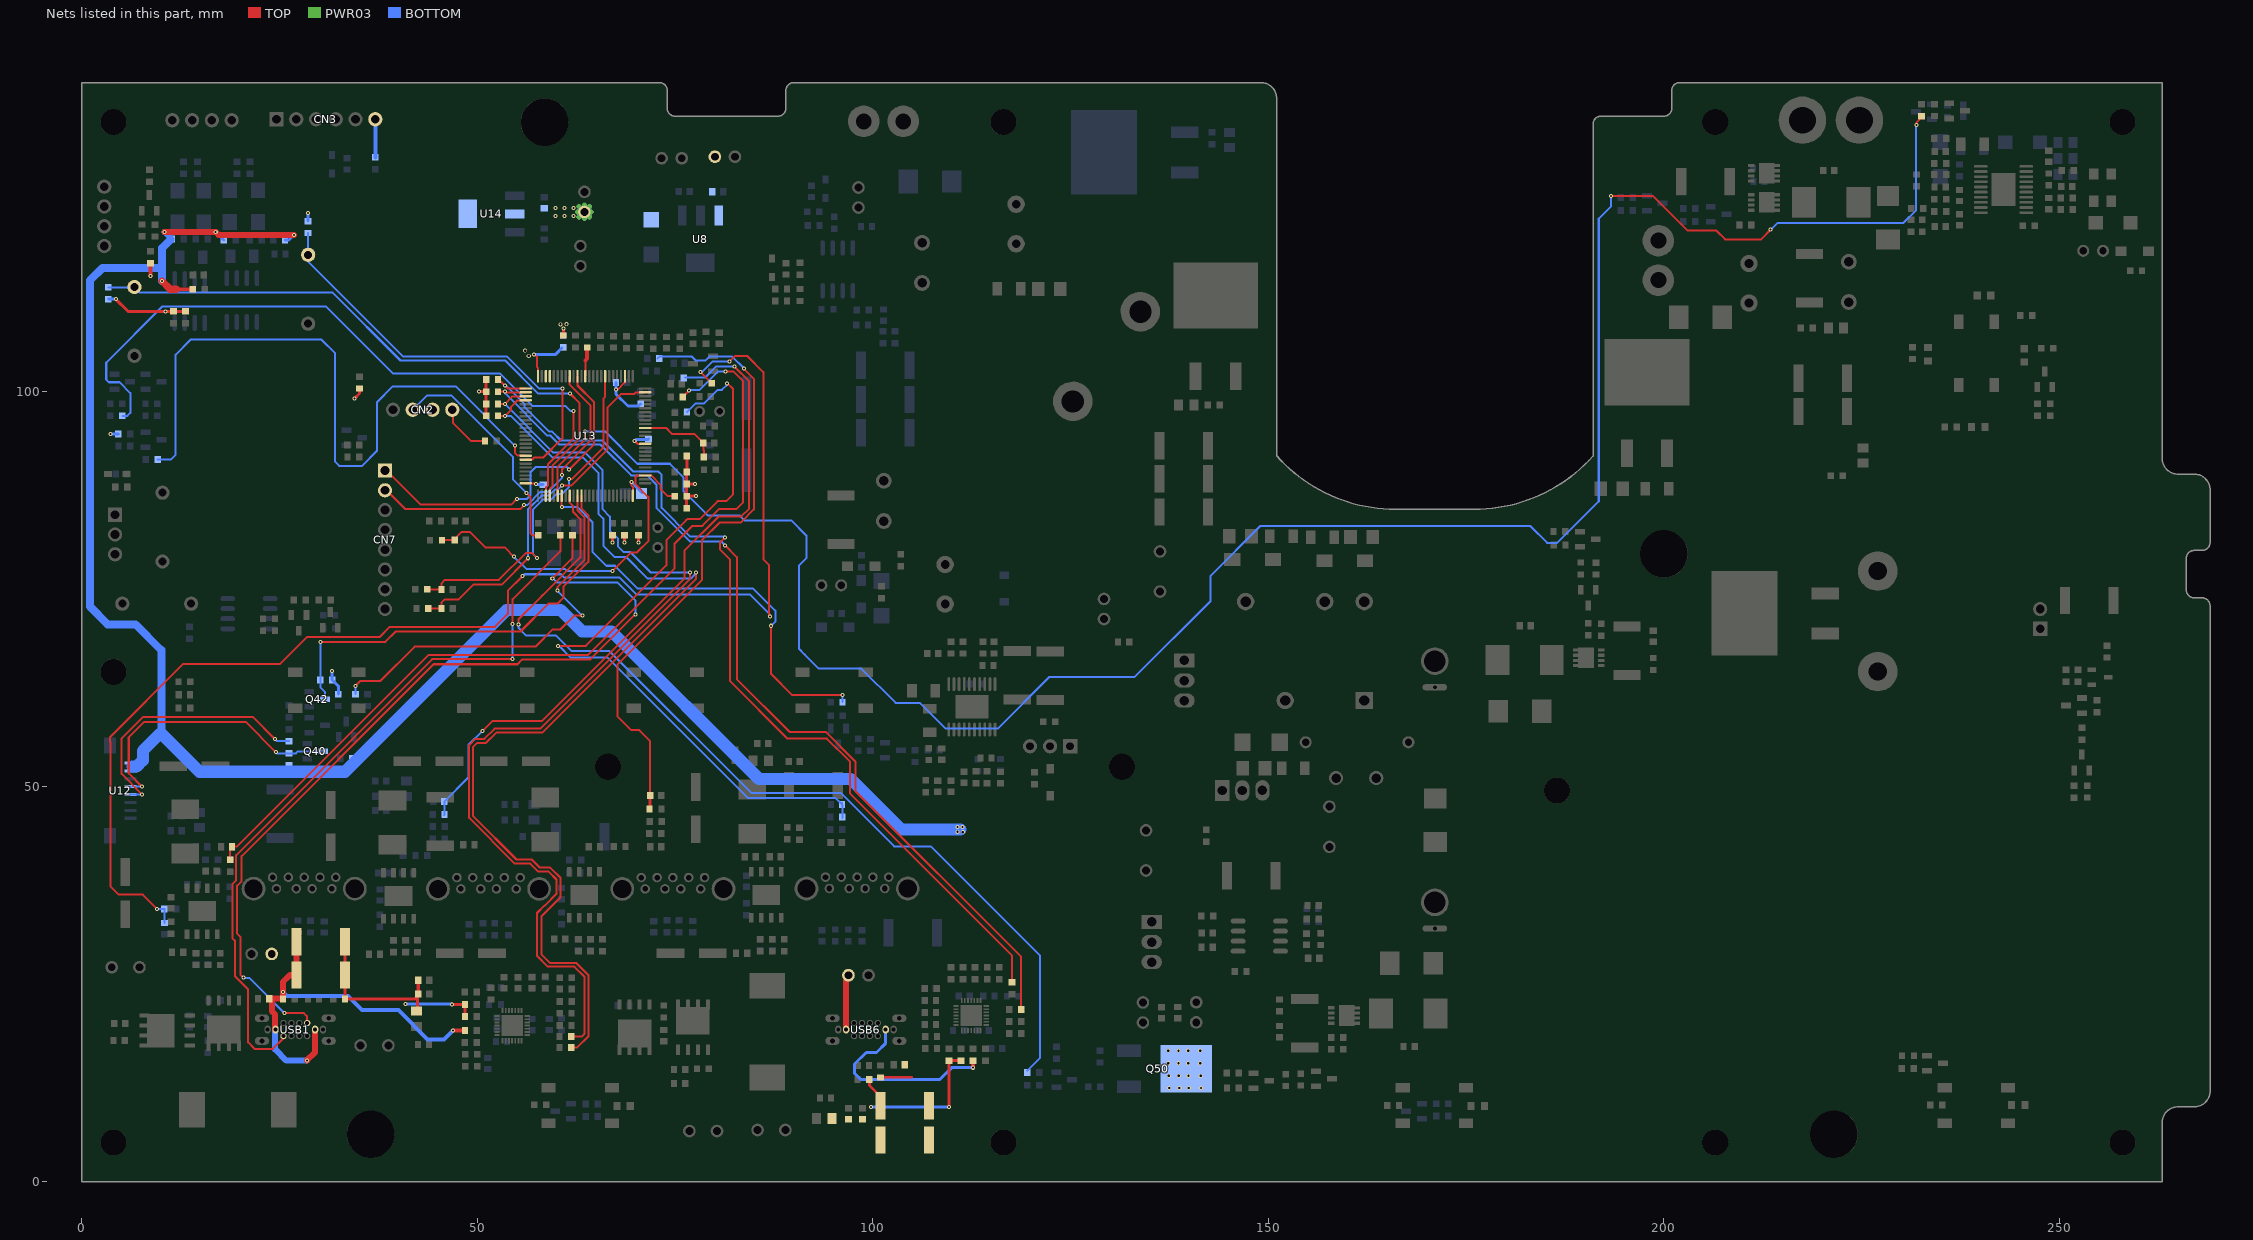
[diagram p0: the nets of this part, all layers, seen from the top]
# Altium PCB MISC84402.PcbDoc (part 9 of 12)
Units mm, origin at the board's own origin, x right, y up, seen from the top; angles counter-clockwise.
Board outline 269.06 x 139 mm, 4 copper layers (TOP, GND02, PWR03, BOTTOM), stack 0.732 mm thick; 694 components, 428 nets, 1859 pads, 1384 vias.

## Via types
v1: diameter 0.508, hole 0.254, TOP to BOTTOM, tented both sides, 1015 vias
v2: diameter 0.508, hole 0.254, TOP to BOTTOM, 243 vias
v3: diameter 0.508, hole 0.305, TOP to BOTTOM, 60 vias
v4: diameter 0.61, hole 0.305, TOP to BOTTOM, 55 vias
v5: diameter 0.61, hole 0.305, TOP to BOTTOM, tented both sides, 8 vias
v6: diameter 0.762, hole 0.381, TOP to BOTTOM, 2 vias
v7: diameter 0.762, hole 0.381, TOP to BOTTOM, tented both sides, 1 vias

## Nets (pads, with @x,y where several pads share a name; then routed paths per layer and width w, separated by ;. In a path a pad name is that pad's centre, name@x,y a point inside that pad or via, vN(x,y) a via of type N, cw(c..) or ccw(c..) an arc to the next point about the centre after c; other vN are vias at no path point) (continued)
NetR349_2: R349.2 U13.84 | length 119
  TOP w0.254: v2@55.194,70.612 55.194,71.145 58.115,74.066 58.242,74.193 63.017,78.969 63.017,83.795 62.103,84.709 62.103,85.446 61.653,85.896 U13.84@61.653,86.776 ; v2(55.22,70.485) v2@55.27,70.536
  BOTTOM w0.254: v2@55.194,70.409 55.194,70.053 56.134,69.113 59.893,69.113 61.9,67.107 66.7,67.107 84.658,49.149 95.987,49.149 102.692,42.443 107.29,42.443 121.133,28.6 121.133,15.697 R349.2@119.507,14.072 ; v2(55.22,70.485) v2@55.296,70.485 ; v2@55.245,70.536 v2@55.296,70.485 ; v2@55.372,70.409 v2@55.296,70.485
"PC UART-RX": R47.1 USB1.B8 | length 109.1
  TOP w0.254: v2@20.422,25.832 20.041,26.213 20.041,30.988 19.634,31.394 19.634,37.465 20.193,38.024 20.193,41.199 44.45,65.456 55.067,65.456 55.677,66.065 64.287,66.065 v1(69.977,71.755) ; v1(25.629,21.361) 25.654,21.336 28.067,21.336 28.48,20.923 USB1.B8@28.48,20.094 ; v1(59.462,76.292) 62.002,78.832 R47.1@62.002,81.77
  BOTTOM w0.254: v2@20.422,25.883 v2@20.447,25.883 ; v2@20.447,25.806 21.158,25.806 v1@25.603,21.361 ; v1@25.616,21.374 v1(25.629,21.361) ; v1@59.589,76.292 60.097,75.784 67.717,75.784 69.977,73.524 v1(69.977,71.755)
  other v2: 20.396,25.832
"PC UART-TX": R324.1 USB1.A8 | length 93.7
  TOP w0.254: USB1.A8@25.48,18.444 25.48,18.19 24.13,16.84 21.819,16.84 21.006,17.653 21.006,24.333 19.355,25.984 19.355,30.48 19.025,30.81 19.025,37.668 19.507,38.151 19.507,41.326 44.272,66.091 v1(54.458,66.091) ; v1(54.458,70.536) 54.458,73.7 60.478,79.721 R324.1@60.478,81.761
  BOTTOM w0.254: v1(54.458,66.091) v1(54.458,70.536) v1@54.458,70.587
POW13.6-EN: R73.1 U13.82 | length 55.4
  TOP w0.254: U13.82@60.653,86.776 60.653,85.397 v1(60.706,85.344) ; v1(87.148,70.323) 87.148,64.227 89.815,61.56 96.205,61.56 v2@96.241,61.595
  BOTTOM w0.254: v1(60.706,85.344) 62.637,85.344 64.542,83.439 64.542,80.95 64.541,79.68 66.311,77.91 67.369,77.91 70.222,75.057 84.827,75.057 87.656,72.228 87.656,70.831 v1(87.148,70.323) ; R73.1@96.156,60.655 v2(96.156,61.586)
POW24-EN: R302.1 U13.81 | length 272.8
  TOP w0.254: U13.81@60.153,86.776 60.153,90.412 63.585,93.845 v1(63.585,94.886) ; v2(193.319,124.638) 198.653,124.638 203.022,120.269 206.654,120.269 207.747,119.177 212.293,119.177 213.538,120.421 v2@213.538,120.447 ; 231.953,133.96 R302.1@232.613,134.62
  BOTTOM w0.254: v1(63.585,94.886) 66.15,94.886 70.231,90.805 74.32,90.805 76.073,89.052 76.073,87.325 79.121,84.277 83.134,84.277 83.757,83.655 89.675,83.655 91.592,81.737 91.592,78.867 90.678,77.953 90.678,67.386 91.389,66.675 ; 91.395,66.681 93.179,64.897 98.552,64.897 102.87,60.579 105.918,60.579 109.195,57.302 115.773,57.302 122.326,63.856 133.096,63.856 142.697,73.457 142.697,76.632 148.996,82.931 183.109,82.931 185.242,80.797 186.512,80.797 191.77,86.055 191.77,121.793 193.294,123.317 193.294,124.638 v2(193.319,124.638) ; v2@213.512,120.396 214.376,121.26 230.302,121.26 231.902,122.86 v2@231.902,133.528
  other v2: 213.462,120.396 231.953,133.655
PV-I: C72.2 R264.1 U13.24 | length 45.9
  TOP w0.254: R264.1@43.797,72.517 C72.2@45.466,72.517 45.466,73.279 45.847,73.66 47.625,73.66 49.496,75.531 53.07,75.531 v1(56.397,78.859) ; v1(60.706,88.076) 61.914,88.076 66.421,92.583 66.421,97.874 68.191,99.644 69.83,99.644 70.012,99.826 U13.24@71.203,99.826
  BOTTOM w0.254: v1(56.397,78.859) 56.397,85.048 58.115,86.766 59.03,86.766 59.792,87.528 60.159,87.528 v1(60.706,88.076)
PV-INT: C69.2 R150.1 R254.1 U13.3 | length 44.8
  TOP w0.254: R254.1@45.745,81.153 C69.2@47.117,81.153 ; C69.2@47.32,81.509 47.981,82.169 49.073,82.169 51.054,80.188 53.492,80.188 v2(54.61,79.07) ; v1(67.056,77.216) 69.444,79.604 70.18,79.604 71.653,81.077 71.653,86.563 71.552,86.665 ; 71.545,86.658 70.012,88.191 70.012,89.189 70.149,89.326 U13.3@71.203,89.326 71.955,89.326 73.178,88.103 73.178,87.595 74.067,86.706 R150.1@74.956,86.706
  BOTTOM w0.254: v2(54.61,79.07) 56.21,77.47 61.087,77.47 61.341,77.216 v1(67.056,77.216)
PV-U: C71.2 R255.1 U13.33 | length 44.7
  TOP w0.254: R255.1@43.67,74.93 C71.2@45.466,74.93 45.466,75.692 45.889,76.115 52.722,76.115 56.151,79.544 56.88,79.544 v1(57.54,78.884) ; v1(61.595,88.9) 61.976,88.9 65.913,92.837 65.913,99.042 66.153,99.282 U13.33@66.153,101.876
  BOTTOM w0.254: v1(57.54,78.884) 57.007,79.417 57.007,84.998 58.318,86.309 59.36,86.309 60.046,86.995 60.706,86.995 61.595,87.884 v1(61.595,88.9)
PWM-H: CN7.2 U13.42 | length 40.3
  TOP w0.254: CN7.2@38.465,87.487 40.845,85.107 55.457,85.107 v1(55.915,85.564) ; v1(60.706,89.408) 60.706,90.127 64.271,93.692 64.271,98.187 61.653,100.806 U13.42@61.653,101.876
  BOTTOM w0.254: v1(55.915,85.564) 56.278,85.564 57.963,87.249 58.928,87.249 60.706,89.027 v1(60.706,89.408)
PWM-L: CN7.1 U13.40 | length 42.7
  TOP w0.254: CN7.1@38.465,89.987 42.811,85.64 54.289,85.64 v1(55,86.352) ; v1(61.595,90.076) 64.77,93.251 64.77,98.577 62.653,100.695 U13.40@62.653,101.876
  BOTTOM w0.254: v1(55,86.352) 56.236,86.352 56.718,86.834 56.718,89.764 57.353,90.399 61.273,90.399 v1(61.595,90.076)
RX_485_INV: D27.2 R158.2 U13.69 | length 54.4
  TOP w0.254: U13.69@56.103,91.326 56.909,91.326 57.15,91.567 58.293,91.567 60.732,94.006 v1(60.732,100.295)
  BOTTOM w0.254: D27.2@28.575,117.043 28.575,116.434 40.65,104.359 53.756,104.359 57.82,100.295 v1(60.732,100.295) ; D27.2@28.601,117.043 R158.2@28.601,119.979
RX_BMS_IN: D26.2 R38.2 U13.79 | length 78.9
  TOP w0.254: U13.79@59.153,86.776 59.153,87.667 59.462,87.976 59.462,90.534 62.891,93.963 62.891,98.501 v1(61.706,99.687)
  BOTTOM w0.254: R38.2@3.328,113.113 6.589,113.113 D26.2@6.63,113.154 7.297,112.487 31.649,112.487 40.275,103.861 53.492,103.861 57.693,99.66 v1@61.706,99.66
RX_BMS_OUT: U13.48
RXD-485: Q40.3 R153.1 U12.4 | length 35.5
  TOP w0.254: v2@7.595,49.987 5.918,51.664 5.918,56.21 7.874,58.166 20.701,58.166 v1(24.511,54.356)
  BOTTOM w0.254: U12.4@6.126,49.979 v2(7.577,49.979) ; v1(24.511,54.356) 24.682,54.185 R153.1@26.188,54.185 27.05,54.185 27.313,54.448 Q40.3@30.49,54.448
RXD-MODBUS: R140.1 U13.86 | length 51.9
  TOP w0.254: v1(34.57,62.703) 35.205,63.338 37.727,63.338 42.072,67.683 57.345,67.683 59.538,69.875 60.503,69.875 62.23,71.603 v1(63.297,71.603) v1@63.373,71.603 ; v1(60.097,74.768) 60.097,75.189 63.526,78.618 63.526,84.039 62.653,84.912 U13.86@62.653,86.776
  BOTTOM w0.254: R140.1@34.57,61.678 v1(34.57,62.703) ; v1(60.097,74.768) 63.262,71.603 v1(63.297,71.603) v1@63.373,71.526
SCK1: R127.2 R249.2 U13.51 | length 117.2
  TOP w0.254: R249.2@52.604,101.438 52.731,101.438 53.468,100.701 v1(53.468,100.676) 53.818,100.326 U13.51@56.103,100.326 ; v1@81.204,81.407 80.645,80.848 80.645,79.985 81.953,78.676 81.953,63.309 89.205,56.058 94.174,56.058 97.13,53.102 97.13,49.098 117.602,28.626 R127.2@117.602,25.264 ; v1@81.209,81.402 v1(81.306,81.499)
  BOTTOM w0.254: v1(53.468,100.676) 53.595,100.549 53.756,100.549 55.969,98.336 55.969,97.945 59.056,94.858 59.452,94.858 60.568,93.743 65.769,93.743 69.686,89.826 72.861,89.826 73.279,89.408 73.279,85.217 76.87,81.626 81.179,81.626 v1(81.306,81.499)
SCK2: R94.2 R199.2 U13.53 | length 128.4
  TOP w0.254: R94.2@52.604,98.339 53.443,98.339 v1(53.493,98.39) 54.429,99.326 U13.53@56.103,99.326 ; 58.471,34.95 57.531,34.011 57.531,28.609 58.908,27.232 62.253,27.232 63.535,25.95 63.535,18.737 63.179,18.381 R199.2@61.884,18.381 ; 58.496,34.925 59.995,36.423 59.995,38.245 58.997,39.243 57.702,39.243 56.686,40.259 54.73,40.259 48.946,46.043 48.946,55.227 49.751,56.032 50.876,56.032 52.172,57.328 57.963,57.328 76.861,76.226 v1(76.861,77.054)
  BOTTOM w0.254: v1(53.493,98.39) 53.493,98.303 59.594,92.202 63.627,92.202 65.786,90.043 65.786,85.09 66.751,84.125 66.751,82.347 67.793,81.305 67.793,80.315 68.453,79.654 69.291,79.654 71.882,77.064 v1@76.733,77.064 ; v1@76.733,77.054 v1(76.861,77.054)
SDA1: R128.2 R246.2 U13.52 | length 118.1
  TOP w0.254: R246.2@52.604,99.914 v1(53.493,99.914) 53.581,99.826 U13.52@56.103,99.826 ; v1(81.306,80.483) 82.804,78.985 82.804,63.551 89.459,56.896 94.054,56.896 97.79,53.16 97.79,49.428 118.745,28.474 R128.2@118.745,21.809
  BOTTOM w0.254: v1(53.493,99.914) 53.493,99.703 58.846,94.35 59.242,94.35 60.357,93.235 65.515,93.235 69.424,89.326 71.456,89.326 72.667,88.115 72.667,85.194 76.87,80.991 80.798,80.991 v1(81.306,80.483)
SDA2: R200.2 R283.2 U13.54 | length 131.5
  TOP w0.254: R283.2@52.604,96.866 v1(53.493,96.866) 54.255,97.627 54.255,98.009 55.072,98.826 U13.54@56.103,98.826 ; R200.2@61.884,16.984 62.577,16.984 64.043,18.45 64.043,26.127 62.467,27.703 59.156,27.703 58.115,28.743 58.115,33.63 60.503,36.017 60.503,38.456 59.207,39.751 57.912,39.751 56.896,40.767 54.94,40.767 49.454,46.253 49.454,55.017 49.962,55.524 51.087,55.524 52.382,56.82 58.217,56.82 77.623,76.226 v1(77.623,77.054)
  BOTTOM w0.254: v1(53.493,96.866) 54.211,96.866 59.468,91.609 63.331,91.609 65.278,89.662 65.278,84.506 65.913,83.871 65.913,80.442 67.31,79.045 68.783,79.045 71.536,76.292 76.952,76.292 v1@77.572,76.911 ; v1@77.623,76.911 v1(77.623,77.054)
SWCLK1: CN2.3 R222.2 | length 28.3
  TOP w0.254: v1(56.194,87.114) 56.727,86.58 56.727,81.981 56.956,81.753 R222.2@57.684,81.753
  BOTTOM w0.254: CN2.3@41.829,97.638 43.632,99.441 46.718,99.441 54.483,91.676 54.483,88.825 v1(56.194,87.114)
SWDIO1: CN2.1 R217.2 | length 6
  TOP w0.254: CN2.1@46.889,96.993 46.889,95.986 49.184,93.691 R217.2@50.962,93.691
TEMP_TC: C126.2 R256.2 U13.15 | length 9.8
  TOP w0.254: U13.15@71.203,95.326 73.848,95.326 74.594,94.58 77.431,94.58 78.566,93.445 78.574,93.437 78.574,92.494 78.648,92.421 R256.2@78.648,91.786
TX_485_INV: R165.1 U13.68 | length 86.8
  TOP w0.254: v1(54.737,93.091) 54.737,92.202 55.113,91.826 U13.68@56.103,91.826
  BOTTOM w0.254: R165.1@9.567,91.33 11.236,91.33 11.837,91.931 11.837,104.613 13.742,106.518 30.252,106.518 32.004,104.766 32.004,91.059 32.512,90.551 35.433,90.551 37.305,92.423 37.305,98.585 39.304,100.584 47.244,100.584 v1(54.737,93.091)
TX_BMS_IN: R159.1 U13.78 | length 89.2
  TOP w0.254: U13.78@58.653,86.776 58.653,87.802 58.954,88.103 58.954,90.774 62.129,93.949 62.129,97.492 v1(62.133,97.496)
  BOTTOM w0.254: R159.1@5.106,96.866 5.741,96.866 6.122,97.247 6.122,99.745 4.758,101.109 3.404,101.109 3.073,101.439 3.073,103.596 10.186,110.709 30.846,110.709 39.355,102.2 52.867,102.2 56.931,98.136 61.113,98.136 61.752,97.496 v1(62.133,97.496)
TX_BMS_OUT: U13.47
TXD-485: R188.2 U12.5 | length 33.1
  TOP w0.254: v2@7.569,49.047 5.029,51.587 5.029,56.083 7.747,58.801 21.59,58.801 v1(24.384,56.007)
  BOTTOM w0.254: U12.5@6.126,48.979 v2(7.577,48.979) ; v1(24.384,56.007) 24.665,55.726 R188.2@26.188,55.726
TXD-MODBUS: Q42.3 R320.1 U13.87 | length 55.1
  TOP w0.254: v1(30.134,68.284) 38.351,68.284 39.663,69.596 55.448,69.596 58.979,73.127 60.122,73.127 60.858,73.863 60.858,74.016 60.859,75.232 64.034,78.407 64.034,84.293 63.153,85.174 U13.87@63.153,86.776
  BOTTOM w0.254: v1(30.134,68.284) R320.1@30.134,63.465 30.134,62.526 30.74,61.92 Q42.3@30.74,61.052
USB-QC-I: C61.2 R77.1 R282.2 | length 167.7
  TOP w0.254: 3.556,55.651 3.556,56.261 12.792,65.497 25.06,65.497 28.448,68.885 37.617,68.885 38.913,70.18 52.197,70.18 53.848,71.832 53.848,74.742 v1(55.724,76.618) ; 3.581,55.651 3.581,37.414 4.674,36.322 7.696,36.322 v2@9.474,34.544 ; v2(78.181,102.412) R282.2@79.612,100.981 ; v2(81.89,103.759) 82.588,104.457 84.087,104.457 86.157,102.387 86.157,78.715 86.894,77.978 86.894,71.593 v1(87.021,71.466)
  BOTTOM w0.254: v2(9.474,34.518) R77.1@10.429,34.518 ; C61.2@10.44,32.733 R77.1@10.44,34.508 ; v1(55.724,76.618) 55.941,76.835 60.57,76.835 60.986,76.419 67.971,76.419 70.094,74.295 84.446,74.295 87.021,71.72 v1(87.021,71.466) ; v2@78.156,102.413 78.182,102.413 78.41,102.413 79.756,103.759 v2(81.89,103.759)
USB-QC-U1: C62.2 R103.2 R280.1 | length 110.9
  TOP w0.254: C62.2@18.745,42.138 R103.2@18.745,40.752 R103.2@18.872,40.879 ; C62.2@18.872,42.138 C62.2@18.872,42.291 ; C62.2@18.949,42.383 C62.2@18.974,42.383 ; C62.2@18.974,42.443 19.634,42.443 43.83,66.64 45.06,66.64 63.998,66.64 74.892,77.534 74.892,80.658 77.191,82.956 78.435,82.956 80.533,85.055 82.703,85.055 83.592,85.944 83.592,101.218 82.321,102.489 v2(81.356,102.489) ; R280.1@75.946,99.247 v2(76.749,100.051)
  BOTTOM w0.254: v2@76.784,100.101 78.054,100.101 80.442,102.489 v2(81.356,102.489)
USB-QC-U2: C46.2 R17.2 R284.2 | length 85.6
  TOP w0.254: v1(50.622,56.998) 51.887,58.262 58.135,58.262 76.162,76.289 76.162,79.784 80.544,84.166 83.381,84.166 84.353,85.138 84.353,99.644 84.353,101.219 v2(82.474,103.099)
  BOTTOM w0.254: R17.2@45.796,46.38 45.811,46.395 C46.2@45.811,48.098 ; C46.2@45.811,48.098 48.87,51.156 48.87,55.245 v1(50.622,56.998) ; R284.2@76.259,101.685 78.775,101.685 80.213,103.124 v2@82.398,103.124 ; v2@82.41,103.06 v2@82.448,103.099
USB-QC-U3: C29.2 R62.2 R285.1 | length 79.4
  TOP w0.254: C29.2@71.843,48.86 71.843,55.742 70.461,57.124 69.445,57.124 67.691,58.878 67.691,65.405 78.384,76.098 78.384,76.784 78.385,81.118 80.671,83.404 83.338,83.404 84.963,85.029 84.963,101.549 v1@83.744,102.768
  TOP w0.381: R62.2@71.79,47.082 R62.2@71.843,47.135 ; R62.2@71.843,47.13 R62.2@71.843,47.135 ; C29.2@71.843,48.86 R62.2@71.843,47.135
  BOTTOM w0.254: R285.1@72.796,104.131 73.059,104.394 77.064,104.394 77.572,103.886 78.867,103.886 79.375,104.394 82.169,104.394 83.769,102.794 v1@83.795,102.794
  other v1: 83.693,102.819
USB-QC-U4: C31.2 R99.2 R286.1 | length 98.8
  TOP w0.254: v1@60.249,67.793 63.714,67.793 73.876,77.955 73.876,81.138 76.405,83.666 ; 76.403,83.668 76.581,83.845 78.156,83.845 80.381,86.071 81.433,86.071 82.322,86.96 82.322,100.253 v2@81.585,100.99
  BOTTOM w0.254: v1@60.325,67.767 61.798,66.294 66.472,66.294 84.226,48.539 95.301,48.539 C31.2@95.987,47.854 ; R286.1@76.504,97.374 77.58,98.45 78.664,98.45 80.366,100.152 80.899,100.152 81.559,100.813 v2(81.559,100.965) v2@81.559,101.016 ; C31.2@96.075,47.942 96.103,47.915 C31.2@96.103,47.717 ; C31.2@96.103,47.646 C31.2@96.103,47.717 ; R99.2@96.13,46.034 R99.2@96.13,46.126 ; R99.2@96.13,46.101 R99.2@96.13,46.126 ; C31.2@96.103,47.717 96.13,47.689 R99.2@96.13,46.126
  other v1: 60.173,67.793
VBUSC-1: C88.2 C189.1 R116.2 R169.2 R179.1 R266.2 USB6.A4 USB6.A9 | length 35.5
  TOP w0.305: R116.2@100.965,13.217 104.911,13.217
  TOP w0.508: v1(112.675,14.443) R179.1@112.675,15.34
  TOP w0.762: USB6.A9@96.621,19.269 96.621,25.704 C189.1@96.901,25.984
  BOTTOM w0.381: USB6.A4@101.621,19.269 101.621,17.547 100.457,16.383 99.162,16.383 97.688,14.91 97.688,13.741 98.476,12.954 108.458,12.954 109.957,14.453 v1@112.674,14.453
VBUSC-2: C141.2 C188.1 R114.2 R216.1 R262.2 R267.2 USB1.A4 USB1.A9 | length 51.4
  TOP w0.508: v1(46.898,19.142) R216.1@48.43,19.142
  TOP w0.762: USB1.A9@24.416,19.206 24.416,19.269 24.416,21.177 24.003,21.59 24.003,23.176 25.355,23.176 R114.2@25.418,23.114 v1(25.418,24.003) 25.418,25.291 26.289,26.162 R267.2@27.141,26.162 R262.2@27.141,30.353 ; v1(28.448,15.367) 29.48,16.399 USB1.A4@29.48,19.269
  BOTTOM w0.508: v1(25.418,24.003) 25.907,23.514 33.616,23.514 35.412,21.717 40.005,21.717 43.688,18.034 45.791,18.034 v1(46.898,19.142)
  BOTTOM w0.762: USB1.A9@24.416,19.206 24.416,16.764 25.838,15.342 v1@28.448,15.342
VCC9V: C78.2 C87.1 CN3.6 R270.1 U8.3 | length 4.8
  BOTTOM w0.508: R270.1@37.091,129.547 CN3.6@37.091,134.366
VDD1: C131.2 C133.2 C137.2 C178.1 R36.2 R237.1 U13.11 U13.28 U13.50 U13.75 U13.100 | length 24.2
  TOP w0.254: U13.75@56.103,88.326 57.334,88.326 v1(57.43,88.23) ; v1@57.15,104.597 v1(57.15,104.648) ; v1@57.226,104.597 57.506,104.318 57.506,103.073 57.653,102.926 U13.50@57.653,101.876 ; v1(67.525,100.168) 67.717,100.168 68.653,101.103 U13.28@68.653,101.876 ; v1(69.469,88.519) 69.469,88.064 69.653,87.88 U13.100@69.653,86.776 ; v1(69.876,93.691) 70.241,93.326 U13.11@71.203,93.326
  BOTTOM w0.381: v1(57.15,104.648) 59.893,104.648 R36.2@60.706,105.461 ; v1(57.43,88.23) 57.495,88.165 C131.2@58.319,88.165 ; C133.2@67.525,101.057 v1(67.525,100.168) 67.525,99.607 69.037,98.095 70.352,98.095 R237.1@70.647,98.39 ; v1(69.469,88.519) 69.469,88.51 70.259,87.719 70.831,87.147 C178.1@70.891,87.147 ; v1(69.876,93.691) 70.068,93.882 70.612,93.882 ; 70.892,93.882 70.612,93.882 ; C137.2@71.628,93.918 71.593,93.882 70.612,93.882
  other v3: 56.49,104.445 56.032,105.105
VDD5V: Q50.3 R144.2 R153.2 R229.2 R231.2 R232.1 R244.1 U12.1 U12.2 | length 233
  TOP w0.381: 11.964,112.868 R229.2@14.013,112.868
  TOP w0.762: v1(10.457,120.107) v1(16.917,120.107) 17.298,119.726 v1(26.823,119.726)
  TOP w0.889: v1(10.135,113.894) 11.161,112.868 11.964,112.868
  BOTTOM w0.381: v1(16.917,120.107) R244.1@17.933,119.091 ; R231.2@25.671,119.091 26.188,119.091 v1(26.823,119.726)
  BOTTOM w0.762: v1(10.457,120.107) R232.1@11.346,119.218 R232.1@11.215,119.087
  BOTTOM w1.016: 9.398,56.54 10.033,57.175 10.033,67.234 6.756,70.51 3.251,70.51 1.016,72.746 1.016,113.995 2.591,115.57 10.084,115.57 ; v1@10.109,113.894 10.109,118.059 R232.1@11.176,119.126
  BOTTOM w1.524: 6.375,52.527 6.909,52.527 7.696,53.315 7.696,54.508 9.728,56.54 10.185,56.54 14.859,51.867 33.249,51.867 53.696,72.314 60.528,72.314 63.221,69.621 66.929,69.621 85.598,50.952 94.158,50.952 94.615,50.952 97.18,50.952 103.556,44.577 111.1,44.577
  other v3: 137.465,11.887 138.735,11.887 139.954,11.887 141.478,11.887 137.414,13.411 138.684,13.411 139.903,13.411 141.427,13.411 137.363,15.011 138.633,15.011 139.852,15.011 141.376,15.011 137.363,16.612 138.633,16.612 139.852,16.612 141.376,16.612 111.379,44.221 110.693,44.272 110.693,44.882 111.328,44.882
"VDD 3.3V": C32.2 C156.1 CN2.2 D14.1 R3.1 R36.1 R38.1 R94.1 R150.2 R152.2 R154.2 R156.2 R157.2 R158.1 R219.2 R221.2 R228.2 R246.1 R249.1 R250.2 R251.2 R252.2 R283.1 R293.2 R319.2 R320.2 R366.2 U14.2 U14.4 | length 51.9
  TOP w0.381: v1(4.291,111.606) 5.824,110.074 R154.2@11.583,110.074 ; v1(10.567,110.073) R156.2@13.107,110.074 ; v1(34.477,99.077) 35.078,99.678 R157.2@35.078,100.312 ; v1(50.191,99.914) R246.1@51.097,99.914 ; R283.1@51.097,96.866 R246.1@51.097,99.914 ; R249.1@51.097,101.438 R246.1@51.097,99.914 ; R3.1@60.859,107.017 v1(60.859,107.915) ; v1(67.082,80.864) R250.2@67.082,81.77 ; v1(68.606,80.864) R251.2@68.606,81.77 ; v1(70.384,80.864) R228.2@70.384,81.77 ; R252.2@76.462,85.182 R150.2@76.462,86.706 ; R293.2@76.471,91.786 76.471,89.763 R221.2@76.462,89.754 R219.2@76.462,88.23 ; v1(77.496,88.23) R219.2@76.462,88.23 ; v1(77.623,86.706) R150.2@76.462,86.706 ; R150.2@76.462,86.706 R219.2@76.462,88.23
  TOP w0.508: v2(8.652,114.545) R366.2@8.652,116.171
  PWR03 w0.635: 62.674,122.647 C156.1@63.526,122.647 ; 62.873,121.994 C156.1@63.526,122.647 ; 62.873,123.299 C156.1@63.526,122.647 ; 63.526,121.795 C156.1@63.526,122.647 ; 63.526,123.498 C156.1@63.526,122.647 ; 64.179,121.994 C156.1@63.526,122.647 ; 64.179,123.299 C156.1@63.526,122.647 ; 64.377,122.647 C156.1@63.526,122.647
  BOTTOM w0.381: R38.1@3.328,111.606 v1(4.291,111.606) ; v1(3.582,94.58) R152.2@4.598,94.58 ; R158.1@28.601,121.486 v1(28.601,122.52) ; v1(31.64,64.599) R320.2@31.64,63.465 32.411,62.694 R319.2@32.411,61.678 ; R36.1@60.859,107.137 v1(60.859,107.915)
  BOTTOM w0.635: 62.674,122.647 C156.1@63.526,122.647 ; 62.873,121.994 C156.1@63.526,122.647 ; 62.873,123.299 C156.1@63.526,122.647 ; 63.526,121.795 C156.1@63.526,122.647 ; 64.179,121.994 C156.1@63.526,122.647 ; 64.179,123.299 C156.1@63.526,122.647 ; 64.377,122.647 C156.1@63.526,122.647
  other v1: 59.843,122.139 60.986,122.139 62.129,122.139 59.843,123.155 60.986,123.155 62.129,123.155
  other v3: 60.503,108.433 61.265,108.458
VOUT1: C83.2 C84.2 L13.2 R115.2 R169.1 R175.1 R178.1 R266.1 | length 21.2
  TOP w0.381: R115.2@99.559,12.954 99.559,12.201 100.954,10.806 R266.1@100.954,9.617 ; v1(109.627,9.49) R175.1@109.627,15.332 ; R175.1@109.644,15.349 R175.1@109.627,15.332 ; R178.1@111.151,15.349 111.133,15.332 R175.1@109.627,15.332
  BOTTOM w0.381: v1(99.736,9.49) v1(109.627,9.49)
VOUT2: C90.2 C138.2 L12.2 R113.2 R214.1 R215.1 R262.1 R267.1 | length 29.4
  TOP w0.381: R262.1@33.274,30.353 R267.1@33.274,26.162 33.274,23.132 R113.2@33.256,23.114 42.062,23.114 C138.2@42.291,23.343 ; L12.2@42.418,21.618 C138.2@42.418,23.749 ; C138.2@42.52,23.749 C90.2@42.52,25.527 ; v1(46.797,22.444) R214.1@48.43,22.444 R215.1@48.43,20.92
  BOTTOM w0.381: v1(40.894,22.479) 46.761,22.479 v1(46.797,22.444)
VREF-EN: R269.2 U13.38 | length 3.7
  TOP w0.254: U13.38@63.653,101.876 63.653,103.886
  TOP w0.508: 63.653,103.886 63.881,104.114 R269.2@63.881,105.51
pads on no net: CN3.3 U1C.5 U1C.27 U1C.28 U2C.5 U2C.27 U2C.28 U12.3 U12.9 U12.10 U13.2 U13.6 U13.7 U13.8 U13.9 U13.37 U13.45 U13.55 U13.56 U13.60 U13.63 U13.65 U13.67 U13.71 U13.91 U13.93 USB1.17 USB2.5 USB2.6 USB2.7 USB2.8 USB2.9 USB2.10 USB2.11 USB3.5 USB3.6 USB3.7 USB3.8 USB3.9 USB3.10 USB3.11 USB4.5 USB4.6 USB4.7 USB4.8 USB4.9 USB4.10 USB4.11 USB5.5 USB5.6 USB5.7 USB5.8 USB5.9 USB5.10 USB5.11 USB6.17 USB6.A8 USB6.B8
copper on no net: | length 1.1
  BOTTOM w0.508: 35.306,129.54 v1(35.306,130.683)

## Polygon pours and split planes (outlines as drawn)
NETQ5_3 on TOP "BottomLayer-No Net" (solid, remove dead copper): 27 vertices, not listed, extent 216.332,73.33 222.631,103.81
GND on TOP "BottomLayer-No Net" (solid, remove dead copper, pour order 1002): 23 vertices, not listed, extent 20.625,21.565 22.682,30.15
VBUSC-2 on TOP "BottomLayer-No Net" (solid, remove dead copper, pour order 1001): 34 vertices, not listed, extent 23.165,18.745 27.864,32.131
+24V on TOP "BottomLayer-No Net" (solid, remove dead copper, pour order 1000): 19 vertices, not listed, extent 50.038,27.762 55.55,29.718
AGND on TOP "BottomLayer-No Net" (solid, remove dead copper, pour order 1001): 18 vertices, not listed, extent 29.972,45.72 35.916,51.054
AGND on TOP "BottomLayer-No Net" (solid, remove dead copper, pour order 1000): 27 vertices, not listed, extent 4.572,37.338 10.668,47.396
GND on TOP "BottomLayer-No Net" (solid, remove dead copper, pour order 1008): 54 vertices, not listed, extent 184.658,18.085 268.554,88.722
+13.6V on TOP "BottomLayer-No Net" (solid, remove dead copper, pour order 1004): 50 vertices, not listed, extent 226.187,56.718 257.708,120.955
GND on TOP "BottomLayer-No Net" (solid, remove dead copper, pour order 1003): 26 vertices, not listed, extent 216.306,114.579 225.628,118.262
+24V on TOP "BottomLayer-No Net" (solid, remove dead copper, pour order 1002): 18 vertices, not listed, extent 216.154,109.88 224.815,112.801
NetQ2_3 on TOP "BottomLayer-No Net" (solid, remove dead copper, pour order 1001): 34 vertices, not listed, extent 140.919,82.144 149.962,103.962
NETC33_1 on TOP "BottomLayer-No Net" (solid, remove dead copper, pour order 1000): 50 vertices, not listed, extent 119.863,73.635 149.2,134.239
+5V on TOP "BottomLayer-No Net" (solid, remove dead copper, pour order 1000): 29 vertices, not listed, extent 87.554,80.086 93.828,108.229
NETCN4_2 on TOP "BottomLayer-No Net" (solid, remove dead copper, pour order 1006): 46 vertices, not listed, extent 3.023,67.996 18.491,88.595
+13.6V on TOP "BottomLayer-No Net" (solid, remove dead copper, pour order 1005): 34 vertices, not listed, extent 93.396,85.954 103.429,105.308
GND on TOP "BottomLayer-No Net" (solid, remove dead copper, pour order 1004): 22 vertices, not listed, extent 93.523,79.426 103.505,84.684
NETC57_2 on TOP "BottomLayer-No Net" (solid, remove dead copper, pour order 1003): 18 vertices, not listed, extent 43.129,48.057 47.117,50.927
NetC105_2 on TOP "BottomLayer-No Net" (solid, remove dead copper, pour order 1002): 22 vertices, not listed, extent 36.17,46.914 43.18,54.94
NetC153_2 on TOP "BottomLayer-No Net" (solid, remove dead copper, pour order 1001): 30 vertices, not listed, extent 76.733,48.108 86.792,54.026
NetC123_2 on TOP "BottomLayer-No Net" (solid, remove dead copper, pour order 1000): 45 vertices, not listed, extent 86.157,44.425 90.373,55.956
BAT1+ on TOP "BottomLayer-No Net" (solid, remove dead copper, pour order 1002): 42 vertices, not listed, extent 155.626,39.954 172.847,62.814
VDD5V on TOP "BottomLayer-No Net" (solid, remove dead copper, pour order 1001): 34 vertices, not listed, extent 110.388,11.328 142.57,45.364
+5V on TOP "BottomLayer-No Net" (solid, remove dead copper, pour order 1015): 42 vertices, not listed, extent 62.001,80.061 91.618,119.482
+12V on TOP "BottomLayer-No Net" (solid, remove dead copper, pour order 1014): 102 vertices, not listed, extent 36.17,66.726 131.42,128.372